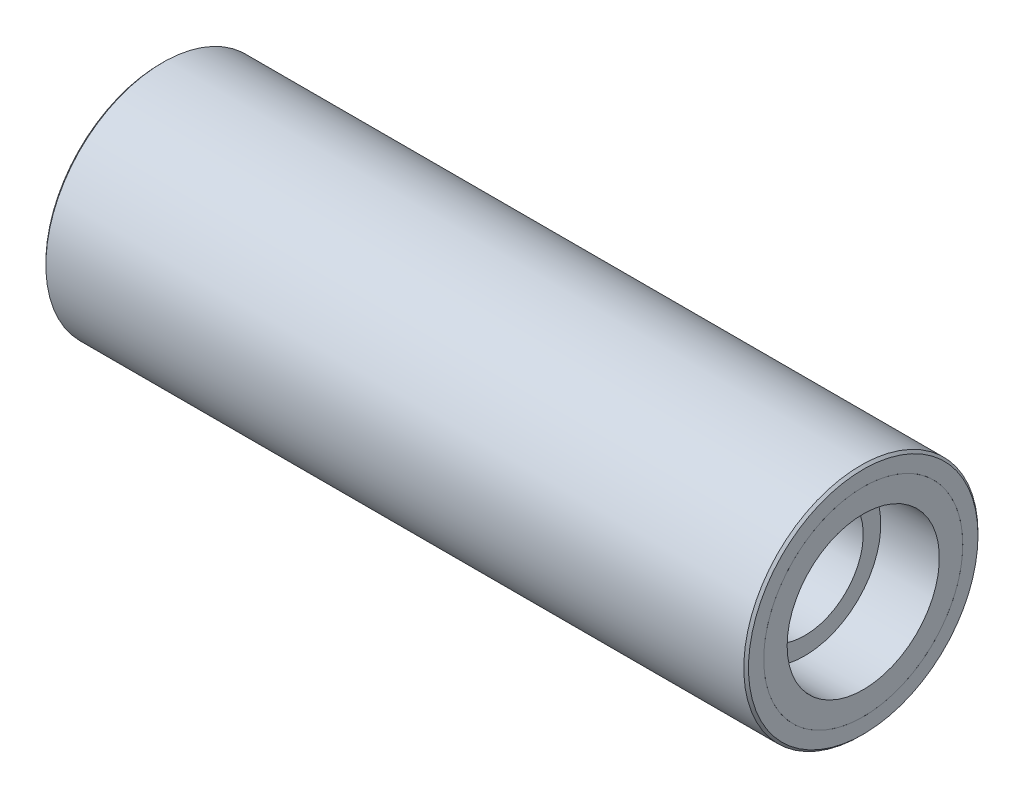
from build123d import *

# Parameters (mm, degrees)
SKETCH2_R           = 10
SKETCH2_R_2         = 8.5
BOSS_EXTRUDE1_DEPTH = 60
CHAMFER1_SIZE       = 0.2


with BuildPart() as part:
    # Sketch1 → Revolve1 (revolve)
    with BuildSketch(Plane.XY, mode=Mode.PRIVATE) as revolve1_sk:
        Polygon((0, 8.5), (60, 8.5), (60, 6.5), (55, 6.5), (55, 5), (5, 5), (5, 6.5), (0, 6.5), align=None)
    revolve(revolve1_sk.sketch.rotate(Axis((0, 0, 0), (1, 0, 0)), 90), axis=Axis((0, 0, 0), (1, 0, 0)))


with BuildPart() as body_2:
    # Sketch2 → Boss-Extrude1 (new body)
    with BuildSketch(Plane(origin=(60, 0, 0), x_dir=(0, 0, -1), z_dir=(1, 0, 0))):
        Circle(SKETCH2_R)
        Circle(SKETCH2_R_2, mode=Mode.SUBTRACT)
    extrude(amount=-BOSS_EXTRUDE1_DEPTH)

    # Chamfer1
    chamfer1_edges = [body_2.edges().sort_by_distance(p)[0] for p in [
        (60, 0, 10),
        (0, 0, 10),
    ]]
    chamfer(chamfer1_edges, length=CHAMFER1_SIZE)


solid = Compound([part.part, body_2.part])
